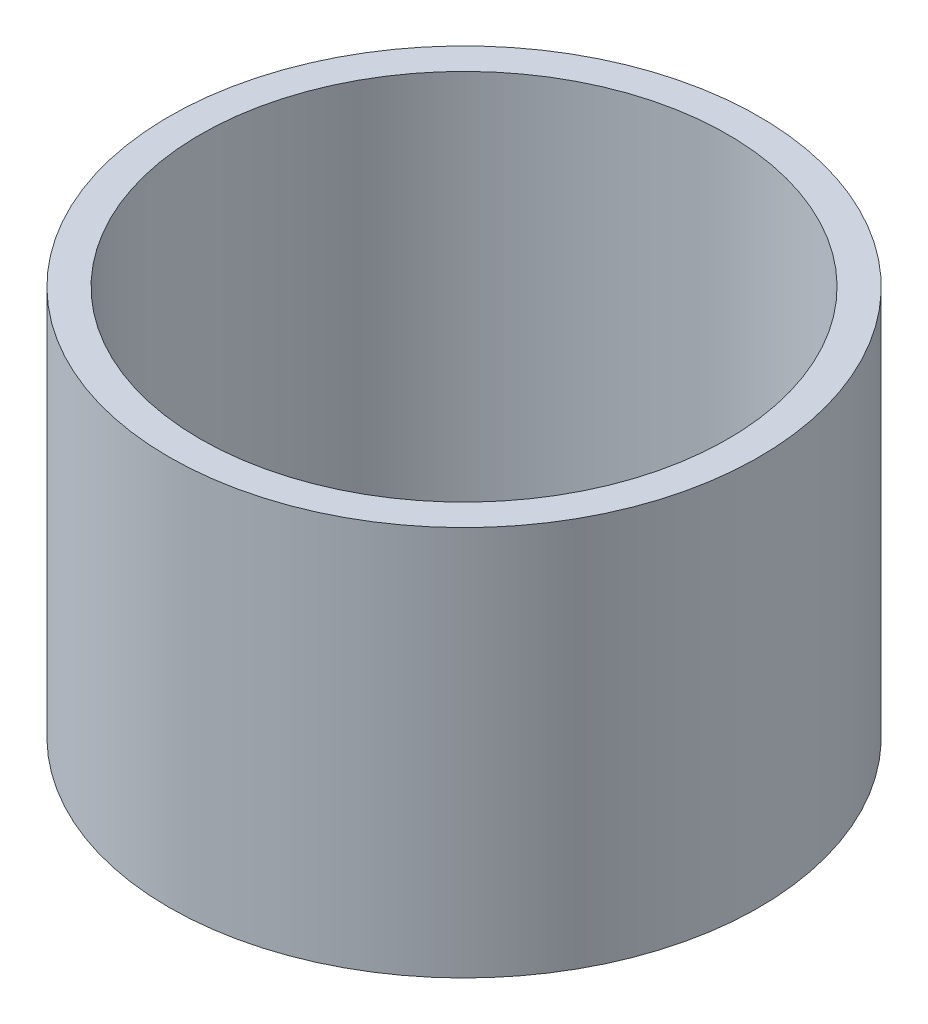
SolidWorks part; units mm, degrees
material "STPG370E"
ref_plane "Front Plane" through (0, 0, 0) normal (0, 0, 1) x (1, 0, 0)
ref_plane "Top Plane" through (0, 0, 0) normal (0, 1, 0) x (1, 0, 0)
ref_plane "Right Plane" through (0, 0, 0) normal (1, 0, 0) x (0, 0, -1)
sketch "Sketch1" plane through (0, 0, 0) normal (0, 1, 0) x (1, 0, 0)
  circle A0 centre (0, 0) radius 30.25
  circle A1 centre (0, 0) radius 27.05
  dimension "D1" = 60.5
  dimension "D2" = 3.2
extrude "Boss-Extrude1" add sketch "Sketch1" along normal blind 40
